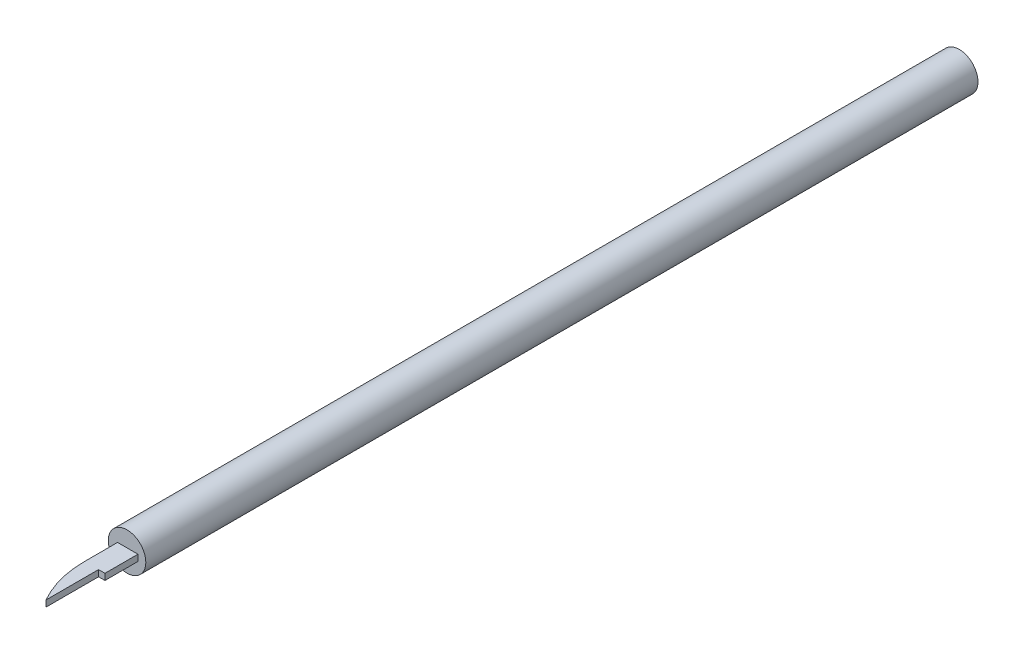
from build123d import *

# Parameters (mm, degrees)
BOSS_EXTRUDE1_DEPTH      = 20
BOSS_EXTRUDE1_DEPTH_BACK = 46
SKETCH1_R                = 1.5
SKETCH2_R                = 1.5
BOSS_EXTRUDE2_DEPTH      = 0.5
BOSS_EXTRUDE3_DEPTH      = 0.25


with BuildPart() as part:
    # Sketch1 → Boss-Extrude1 (new, two sides: drawn at the far end of the back side and taken through both)
    with BuildSketch(Plane.XY.offset(-BOSS_EXTRUDE1_DEPTH_BACK)):
        Circle(SKETCH1_R)
    extrude(amount=BOSS_EXTRUDE1_DEPTH + BOSS_EXTRUDE1_DEPTH_BACK)

    # Sketch2 → Boss-Extrude2 (add)
    with BuildSketch(Plane.XY.offset(20)):
        Circle(SKETCH2_R)
    extrude(amount=BOSS_EXTRUDE2_DEPTH)

    # Sketch3 → Boss-Extrude3 (add, symmetric)
    with BuildSketch(Plane(origin=(0, 0, 0), x_dir=(1, 0, 0), z_dir=(0, 1, 0))):
        with BuildLine():
            Line((0.873889529, -20.5), (-0.757865329, -20.5))
            Line((-0.757865329, -20.5), (-0.757865329, -23.138895886))
            ThreePointArc((-0.757865329, -23.138895886), (-0.472929345, -25.311777544), (0.362611115, -27.337728025))
            Line((0.362611115, -27.337728025), (0.362611115, -23.138895886))
            Line((0.362611115, -23.138895886), (0.873889529, -23.138895886))
            Line((0.873889529, -23.138895886), (0.873889529, -20.5))
        make_face()
    extrude(amount=BOSS_EXTRUDE3_DEPTH, both=True)


solid = part.part
